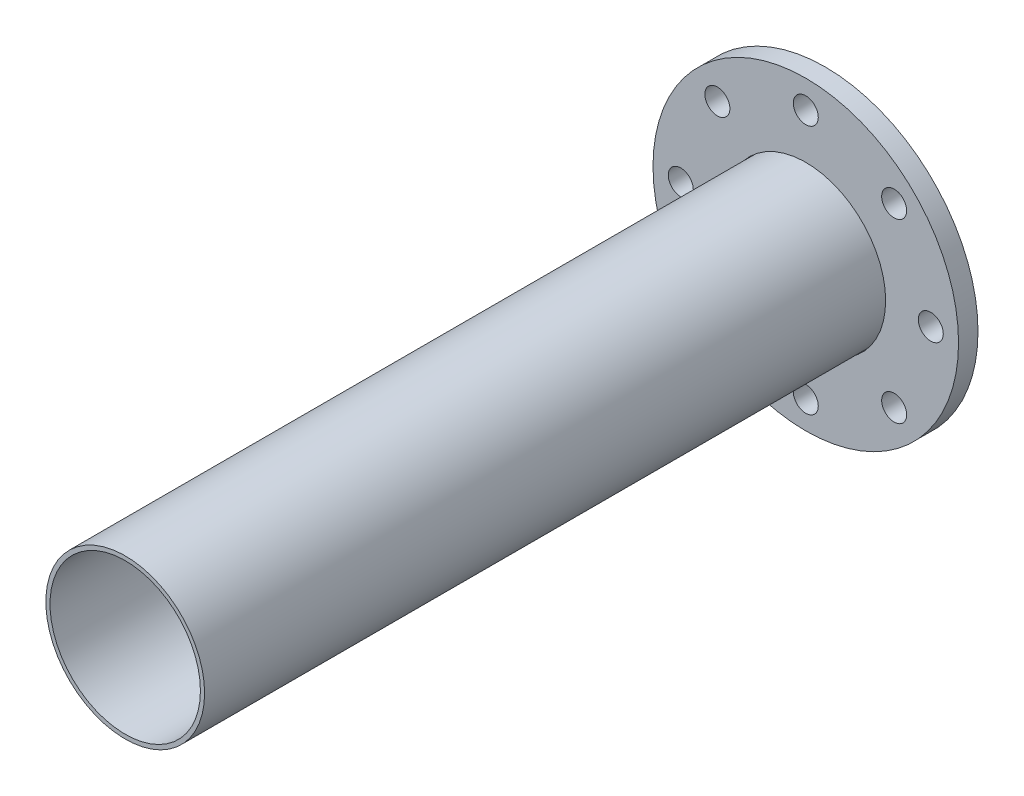
SolidWorks part; units mm, degrees
material "Plain carbon steel"
ref_plane "Front Plane" through (0, 0, 0) normal (0, 0, 1) x (1, 0, 0)
ref_plane "Top Plane" through (0, 0, 0) normal (0, 1, 0) x (1, 0, 0)
ref_plane "Right Plane" through (0, 0, 0) normal (1, 0, 0) x (0, 0, -1)
sketch "Sketch1" plane through (0, 0, 0) normal (0, 0, 1) x (1, 0, 0)
  circle A0 centre (0, 0) radius 110
  circle A1 centre (0, 0) radius 90 construction
  circle A2 centre (0, 0) radius 57.5
  circle A3 centre (0, 90) radius 9
  circle A4 centre (63.6396, 63.6396) radius 9
  circle A5 centre (90, 0) radius 9
  circle A6 centre (63.6396, -63.6396) radius 9
  circle A7 centre (0, -90) radius 9
  circle A8 centre (-63.6396, -63.6396) radius 9
  circle A9 centre (-90, 0) radius 9
  circle A10 centre (-63.6396, 63.6396) radius 9
  dimension "D1" = 115
  dimension "D2" = 180
  dimension "D3" = 220
  dimension "D4" = 18
  dimension "D5" = 8
extrude "Boss-Extrude1" add sketch "Sketch1" along normal blind 14
ref_plane "Plane1" through (0, 0, 4) normal (0, 0, 1) x (1, 0, 0)
sketch "Sketch2" plane through (0, 0, 4) normal (0, 0, 1) x (1, 0, 0)
  circle A0 centre (0, 0) radius 57.15
  circle A1 centre (0, 0) radius 54.15
  dimension "D1" = 114.3
  dimension "D2" = 3
extrude "Boss-Extrude2" add sketch "Sketch2" along normal blind 500 separate body
sketch "Sketch3" plane through (0, 0, 0) normal (0, 0, -1) x (-1, 0, 0)
  line L0 (0, 0) -> (0, 90) construction
  line L1 (0, 90) -> (90, 0) construction
  line L2 (90, 0) -> (0, 0) construction
  line L3 (0, 90) -> (63.6396, 63.6396) construction
  line L4 (63.6396, 63.6396) -> (0, 0) construction
  line L5 (0, 0) -> (31.8198, 76.8198) construction
  line L6 (31.8198, 76.8198) -> (48.3829, 116.8066) construction
